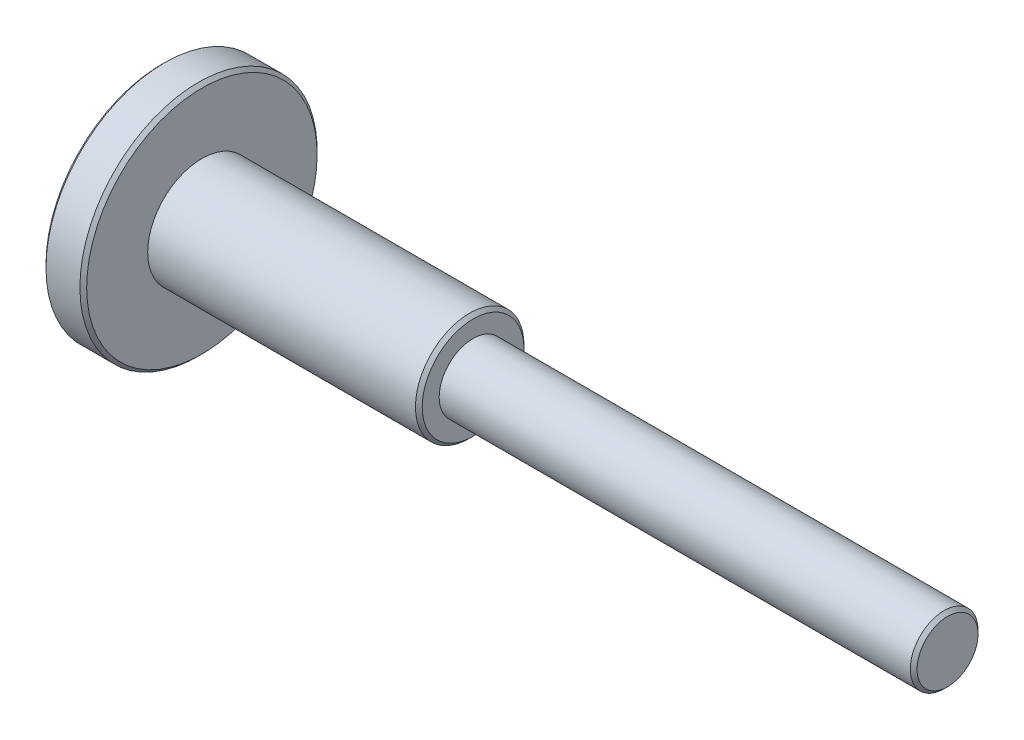
from build123d import *

# Parameters (mm, degrees)
CHAMFER1_SIZE = 0.5
CHAMFER2_SIZE = 0.5


with BuildPart() as part:
    # Sketch1 → Revolve1 (revolve)
    with BuildSketch(Plane.XY, mode=Mode.PRIVATE) as revolve1_sk:
        Polygon((0, 0), (0, 17.5), (6, 17.5), (6, 8), (46, 8), (46, 5), (116, 5), (116, 0), align=None)
    revolve(revolve1_sk.sketch.rotate(Axis((0, 0, 0), (1, 0, 0)), 90), axis=Axis((0, 0, 0), (1, 0, 0)))

    # Chamfer1
    chamfer1_edges = [part.edges().sort_by_distance(p)[0] for p in [
        (46, 0, -8),
        (6, 0, -17.5),
        (0, 0, -17.5),
    ]]
    chamfer(chamfer1_edges, length=CHAMFER1_SIZE)

    # Chamfer2
    chamfer2_edges = [part.edges().sort_by_distance(p)[0] for p in [
        (116, 0, -5),
    ]]
    chamfer(chamfer2_edges, length=CHAMFER2_SIZE)


solid = part.part
